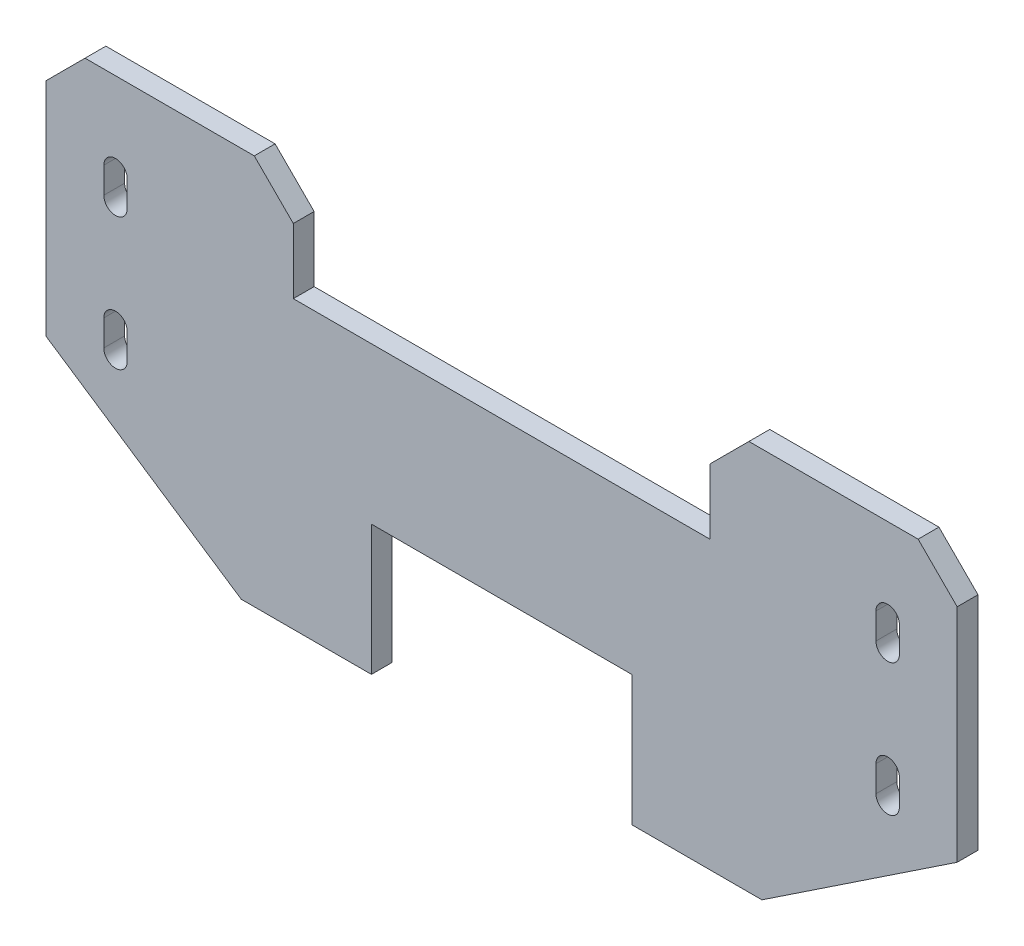
SolidWorks part; units mm, degrees
material "1023 碳钢板 (SS)"
ref_plane "前视基准面" through (0, 0, 0) normal (0, 0, 1) x (1, 0, 0)
ref_plane "上视基准面" through (0, 0, 0) normal (0, 1, 0) x (1, 0, 0)
ref_plane "右视基准面" through (0, 0, 0) normal (1, 0, 0) x (0, 0, -1)
sketch "草图1" plane through (0, 0, 0) normal (0, 0, 1) x (1, 0, 0)
  line L0 (175, -25) -> (100, -75)
  line L1 (-160, 75) -> (-95, 75)
  line L2 (-175, 60) -> (-175, -25)
  line L3 (-100, -75) -> (-50, -75)
  line L4 (175, 60) -> (175, -25)
  line L5 (-175, 75) -> (175, -75) construction
  line L6 (-175, -75) -> (175, 75) construction
  line L7 (-175, -25) -> (-100, -75)
  line L8 (-50, -75) -> (-50, -25)
  line L9 (-50, -25) -> (50, -25)
  line L10 (50, -25) -> (50, -75)
  line L11 (-175, 60) -> (-160, 75)
  line L12 (160, 75) -> (175, 60)
  line L13 (95, 75) -> (160, 75)
  line L15 (-80, 60) -> (-80, 35)
  line L16 (-80, 35) -> (80, 35)
  line L17 (80, 60) -> (80, 35)
  line L18 (-148.3, 43) -> (-148.3, 33) construction
  line L19 (-143.8, 43) -> (-143.8, 33)
  line L20 (50, -75) -> (100, -75)
  line L21 (-95, 75) -> (-80, 60)
  line L22 (95, 75) -> (80, 60)
  line L23 (-152.8, 43) -> (-152.8, 33)
  line L24 (-148.3, -7.8) -> (-148.3, -17.8) construction
  line L25 (-143.8, -7.8) -> (-143.8, -17.8)
  line L26 (-152.8, -7.8) -> (-152.8, -17.8)
  line L27 (0, 0) -> (0, 66.932) construction
  line L28 (148.3, -7.8) -> (148.3, -17.8) construction
  line L29 (143.8, -7.8) -> (143.8, -17.8)
  line L30 (152.8, -7.8) -> (152.8, -17.8)
  line L31 (148.3, 43) -> (148.3, 33) construction
  line L32 (143.8, 43) -> (143.8, 33)
  line L33 (152.8, 43) -> (152.8, 33)
  arc A0 (-143.8, 43) -> (-152.8, 43) centre (-148.3, 43) ccw
  arc A1 (-152.8, 33) -> (-143.8, 33) centre (-148.3, 33) ccw
  arc A2 (-143.8, -7.8) -> (-152.8, -7.8) centre (-148.3, -7.8) ccw
  arc A3 (-152.8, -17.8) -> (-143.8, -17.8) centre (-148.3, -17.8) ccw
  arc A4 (143.8, -7.8) -> (152.8, -7.8) centre (148.3, -7.8) cw
  arc A5 (152.8, -17.8) -> (143.8, -17.8) centre (148.3, -17.8) cw
  arc A6 (143.8, 43) -> (152.8, 43) centre (148.3, 43) cw
  arc A7 (152.8, 33) -> (143.8, 33) centre (148.3, 33) cw
  point P0 (0, 0)
  point P12 (0, -25)
  point P21 (-148.3, 38)
  point P24 (-80, 75)
  point P25 (80, 75)
  point P34 (-148.3, -12.8)
  point P45 (148.3, -12.8)
  point P52 (148.3, 38)
  point P57 (0, 0)
  point P58 (0, 0)
  dimension "D14" = 4.5
  dimension "D1" = 350
  dimension "D2" = 150
  dimension "D3" = 75
  dimension "D4" = 75
  dimension "D5" = 50
  dimension "D6" = 50
  dimension "D7" = 100
  dimension "D8" = 50
  dimension "D9" = 15
  dimension "D10" = 45
  dimension "D11" = 15
  dimension "D12" = 45
  dimension "D13" = 10
  dimension "D15" = 50.8
  dimension "D16" = 160
  dimension "D19" = 25
  dimension "D20" = 50
  dimension "D21" = 32
  dimension "D22" = 26.7
extrude "凸台-拉伸1" add sketch "草图1" along normal blind 8
